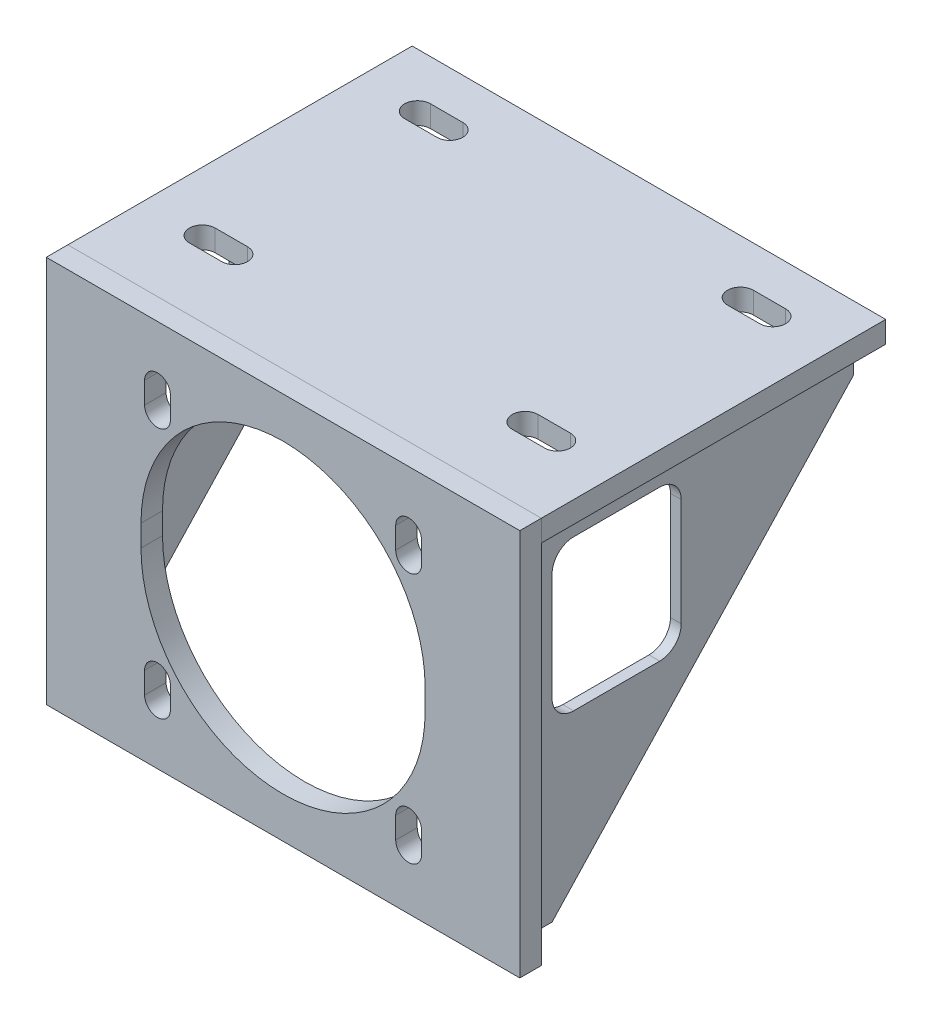
SolidWorks part; units mm, degrees
material "Q235-A"
ref_plane "Front Plane" through (0, 0, 0) normal (0, 0, 1) x (1, 0, 0)
ref_plane "Top Plane" through (0, 0, 0) normal (0, 1, 0) x (1, 0, 0)
ref_plane "Right Plane" through (0, 0, 0) normal (1, 0, 0) x (0, 0, -1)
sketch "Sketch1" plane through (0, 0, 0) normal (0, 0, 1) x (1, 0, 0)
  line L1 (-110, 90) -> (110, 90)
  line L2 (-110, 90) -> (-110, -90)
  line L3 (-110, -90) -> (110, -90)
  line L4 (110, 90) -> (110, -90)
  line L5 (0, -90) -> (0, 90) construction
  line L6 (-110, 0) -> (110, 0) construction
  point P0 (0, 0)
  dimension "D1" = 220
  dimension "D2" = 180
extrude "Boss-Extrude1" add sketch "Sketch1" along normal mid plane 10
sketch "Sketch2" plane through (0, 0, -5) normal (0, 0, -1) x (-1, 0, 0)
  line L0 (110, -90) -> (-110, -90) construction
  line L2 (0, 0) -> (0, -90) construction
  circle A0 centre (0, 0) radius 65.5
  dimension "D1" = 131
  dimension "D2" = 90
extrude "Cut-Extrude1" cut sketch "Sketch2" against normal blind 55
sketch "Sketch3" plane through (0, 0, -5) normal (0, 0, -1) x (-1, 0, 0)
  line L0 (0, 0) -> (-58.3363, 58.3363) construction
  line L1 (0, 0) -> (-147.248, 0) construction
  circle A0 centre (0, 0) radius 82.5 construction
  circle A1 centre (0, 0) radius 65.5 construction
  circle A2 centre (-58.3363, 58.3363) radius 5.5
  dimension "D1" = 165
  dimension "D3" = 11
  dimension "D2" = 45
extrude "Cut-Extrude2" cut sketch "Sketch3" against normal blind 55
pattern_circular "CirPattern1" count 4 over 360 about axis through (0, 0, 0) along (0, 0, 1) of "Cut-Extrude2"
sketch "Sketch4" plane through (0, 0, -5) normal (0, 0, -1) x (-1, 0, 0)
  line L0 (-110, -90) -> (-110, 90) construction
  line L1 (110, 90) -> (-110, 90)
  line L2 (110, 90) -> (110, 80)
  line L3 (110, 80) -> (-110, 80)
  line L4 (-110, 90) -> (-110, 80)
  dimension "D1" = 10
extrude "Boss-Extrude2" add sketch "Sketch4" along normal blind 160 separate body
sketch "Sketch6" plane through (-110, 0, 0) normal (-1, 0, 0) x (0, 0, 1)
  line L0 (-5, 70) -> (-5, -80)
  line L1 (-5, 90) -> (-5, -90) construction
  line L2 (-5, -80) -> (-15, -80)
  line L3 (-15, -80) -> (-155, 70)
  line L4 (-155, 70) -> (-155, 80)
  line L5 (-165, 80) -> (-5, 80) construction
  line L6 (-155, 80) -> (-15, 80)
  line L7 (-15, 80) -> (-5, 70)
  dimension "D1" = 10
  dimension "D2" = 10
  dimension "D3" = 150
  dimension "D4" = 150
  dimension "D5" = 10
  dimension "D6" = 10
extrude "Boss-Extrude3" add sketch "Sketch6" against normal blind 5 from offset 5 separate body offset against normal yes
mirror "Mirror1" about plane through (0, 0, 0) normal (1, 0, 0) of bodies 115
sketch "Sketch7" plane through (0, 0, 5) normal (0, 0, 1) x (1, 0, 0)
  line L0 (-58.3363, 63.3363) -> (-58.3363, 53.3363) construction
  line L1 (-52.3363, 63.3363) -> (-52.3363, 53.3363)
  line L2 (-64.3363, 63.3363) -> (-64.3363, 53.3363)
  line L3 (58.3363, 63.3363) -> (58.3363, 53.3363) construction
  line L4 (64.3363, 63.3363) -> (64.3363, 53.3363)
  line L5 (52.3363, 63.3363) -> (52.3363, 53.3363)
  line L6 (58.3363, -63.3363) -> (58.3363, -53.3363) construction
  line L7 (52.3363, -63.3363) -> (52.3363, -53.3363)
  line L8 (64.3363, -63.3363) -> (64.3363, -53.3363)
  line L9 (-58.3363, -53.3363) -> (-58.3363, -63.3363) construction
  line L10 (-52.3363, -53.3363) -> (-52.3363, -63.3363)
  line L11 (-64.3363, -53.3363) -> (-64.3363, -63.3363)
  arc A0 (-52.3363, 63.3363) -> (-64.3363, 63.3363) centre (-58.3363, 63.3363) ccw
  arc A1 (-64.3363, 53.3363) -> (-52.3363, 53.3363) centre (-58.3363, 53.3363) ccw
  arc A2 (64.3363, 63.3363) -> (52.3363, 63.3363) centre (58.3363, 63.3363) ccw
  arc A3 (52.3363, 53.3363) -> (64.3363, 53.3363) centre (58.3363, 53.3363) ccw
  arc A4 (52.3363, -63.3363) -> (64.3363, -63.3363) centre (58.3363, -63.3363) ccw
  arc A5 (64.3363, -53.3363) -> (52.3363, -53.3363) centre (58.3363, -53.3363) ccw
  arc A6 (-52.3363, -53.3363) -> (-64.3363, -53.3363) centre (-58.3363, -53.3363) ccw
  arc A7 (-64.3363, -63.3363) -> (-52.3363, -63.3363) centre (-58.3363, -63.3363) ccw
  point P2 (-58.3363, 58.3363)
  point P10 (58.3363, 58.3363)
  point P18 (58.3363, -58.3363)
  point P26 (-58.3363, -58.3363)
  dimension "D1" = 6
  dimension "D3" = 6
  dimension "D6" = 6
  dimension "D7" = 6
  dimension "D2" = 10
  dimension "D4" = 10
  dimension "D5" = 10
  dimension "D8" = 10
extrude "Cut-Extrude3" cut sketch "Sketch7" against normal blind 15
sketch "Sketch8" plane through (0, 0, 5) normal (0, 0, 1) x (1, 0, 0)
  line L0 (0, 5) -> (0, -5) construction
  line L1 (66, 5) -> (66, -5)
  line L2 (-66, 5) -> (-66, -5)
  arc A0 (66, 5) -> (-66, 5) centre (0, 5) ccw
  arc A1 (-66, -5) -> (66, -5) centre (0, -5) ccw
  point P2 (0, 0)
  dimension "D2" = 66
  dimension "D1" = 10
extrude "Cut-Extrude4" cut sketch "Sketch8" against normal blind 16
sketch "Sketch9" plane through (0, 80, 0) normal (0, -1, 0) x (1, 0, 0)
  line L0 (67.5, -40) -> (82.5, -40) construction
  line L1 (67.5, -34) -> (82.5, -34)
  line L2 (67.5, -46) -> (82.5, -46)
  line L3 (-110, -5) -> (110, -5) construction
  arc A0 (67.5, -34) -> (67.5, -46) centre (67.5, -40) ccw
  arc A1 (82.5, -46) -> (82.5, -34) centre (82.5, -40) ccw
  point P2 (75, -40)
  dimension "D1" = 6
  dimension "D2" = 15
  dimension "D3" = 75
  dimension "D4" = 35
extrude "Cut-Extrude5" cut sketch "Sketch9" against normal blind 16
pattern_linear "LPattern1" count 2 spacing 150 along (-1, 0, 0) count 2 spacing 100 along (0, 0, -1) of "Cut-Extrude5"
sketch "Sketch10" plane through (-105, 0, 0) normal (-1, 0, 0) x (0, 0, 1)
  line L0 (-5, 90) -> (-5, -90) construction
  line L1 (-65, 70) -> (-25, 70)
  line L2 (-75, 60) -> (-75, 10)
  line L3 (-65, 0) -> (-25, 0)
  line L4 (-15, 60) -> (-15, 10)
  line L5 (-15, 80) -> (-155, 80) construction
  arc A0 (-65, 70) -> (-75, 60) centre (-65, 60) ccw
  arc A1 (-65, 0) -> (-75, 10) centre (-65, 10) cw
  arc A2 (-25, 0) -> (-15, 10) centre (-25, 10) ccw
  arc A3 (-15, 60) -> (-25, 70) centre (-25, 60) ccw
  point P10 (-75, 70)
  point P13 (-75, 0)
  point P18 (-15, 70)
  dimension "D5" = 10
  dimension "D1" = 10
  dimension "D2" = 60
  dimension "D3" = 10
  dimension "D4" = 70
extrude "Cut-Extrude6" cut sketch "Sketch10" against normal blind 317
